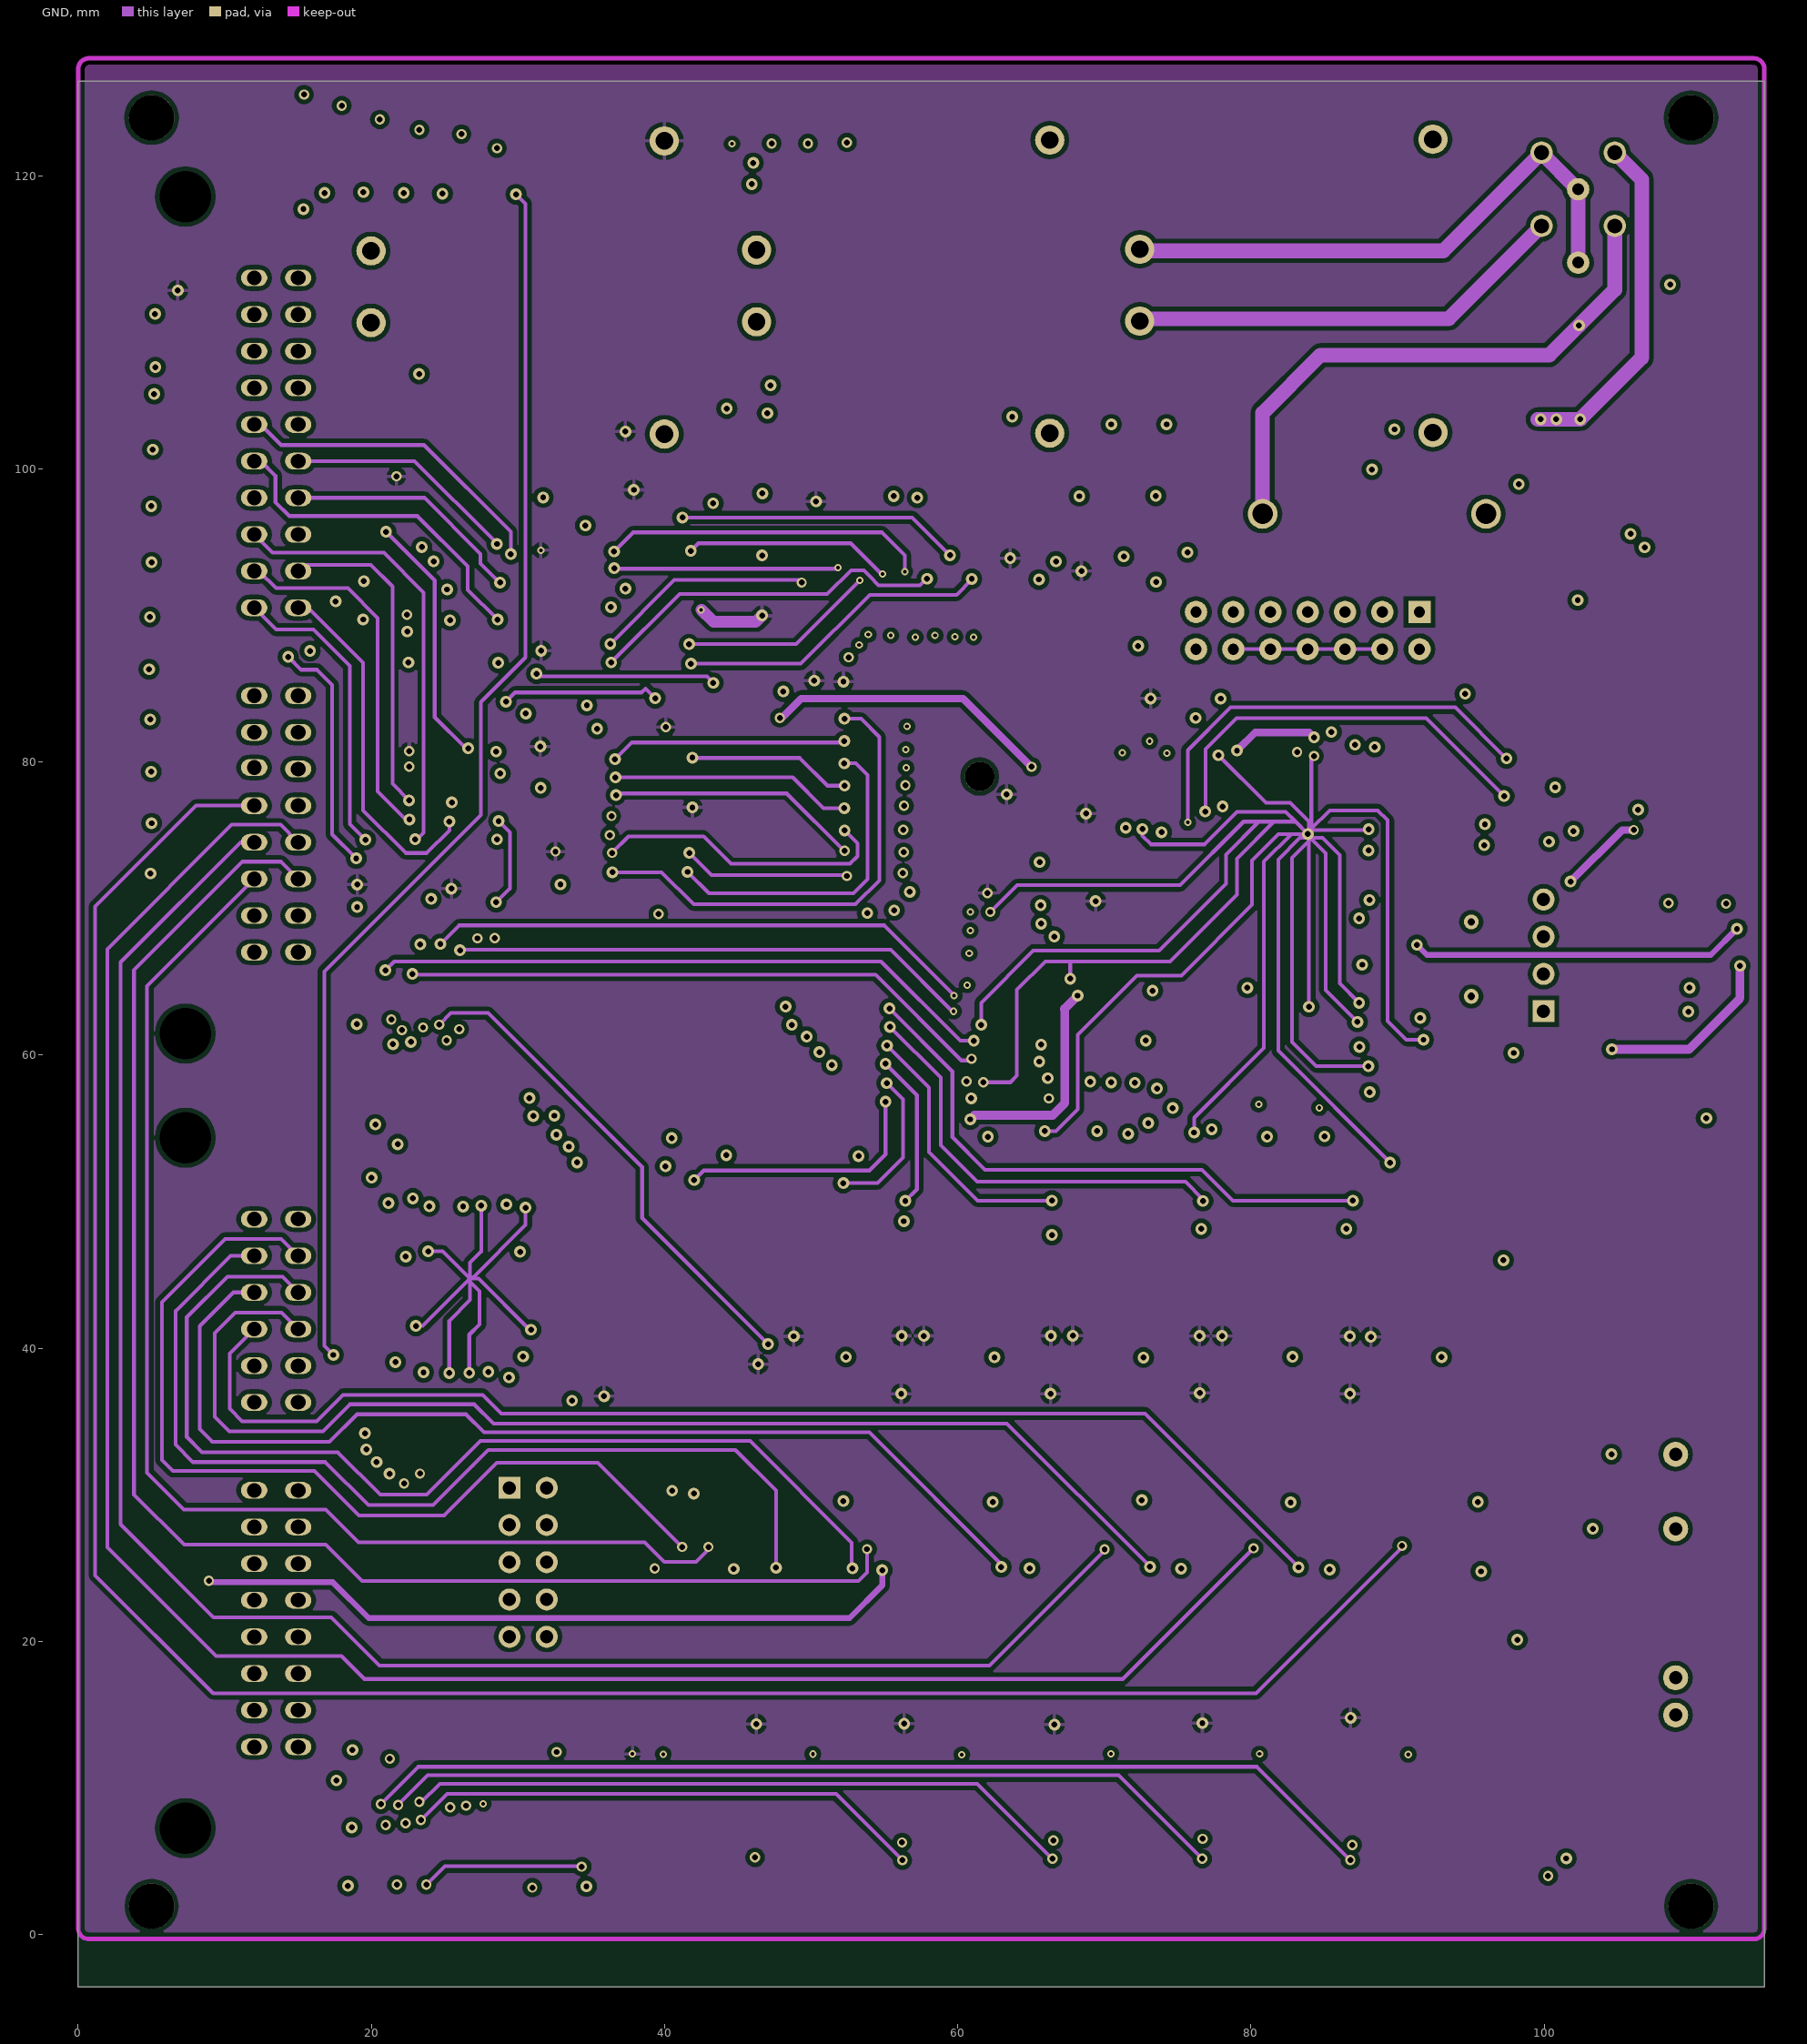
[diagram p0: GND]
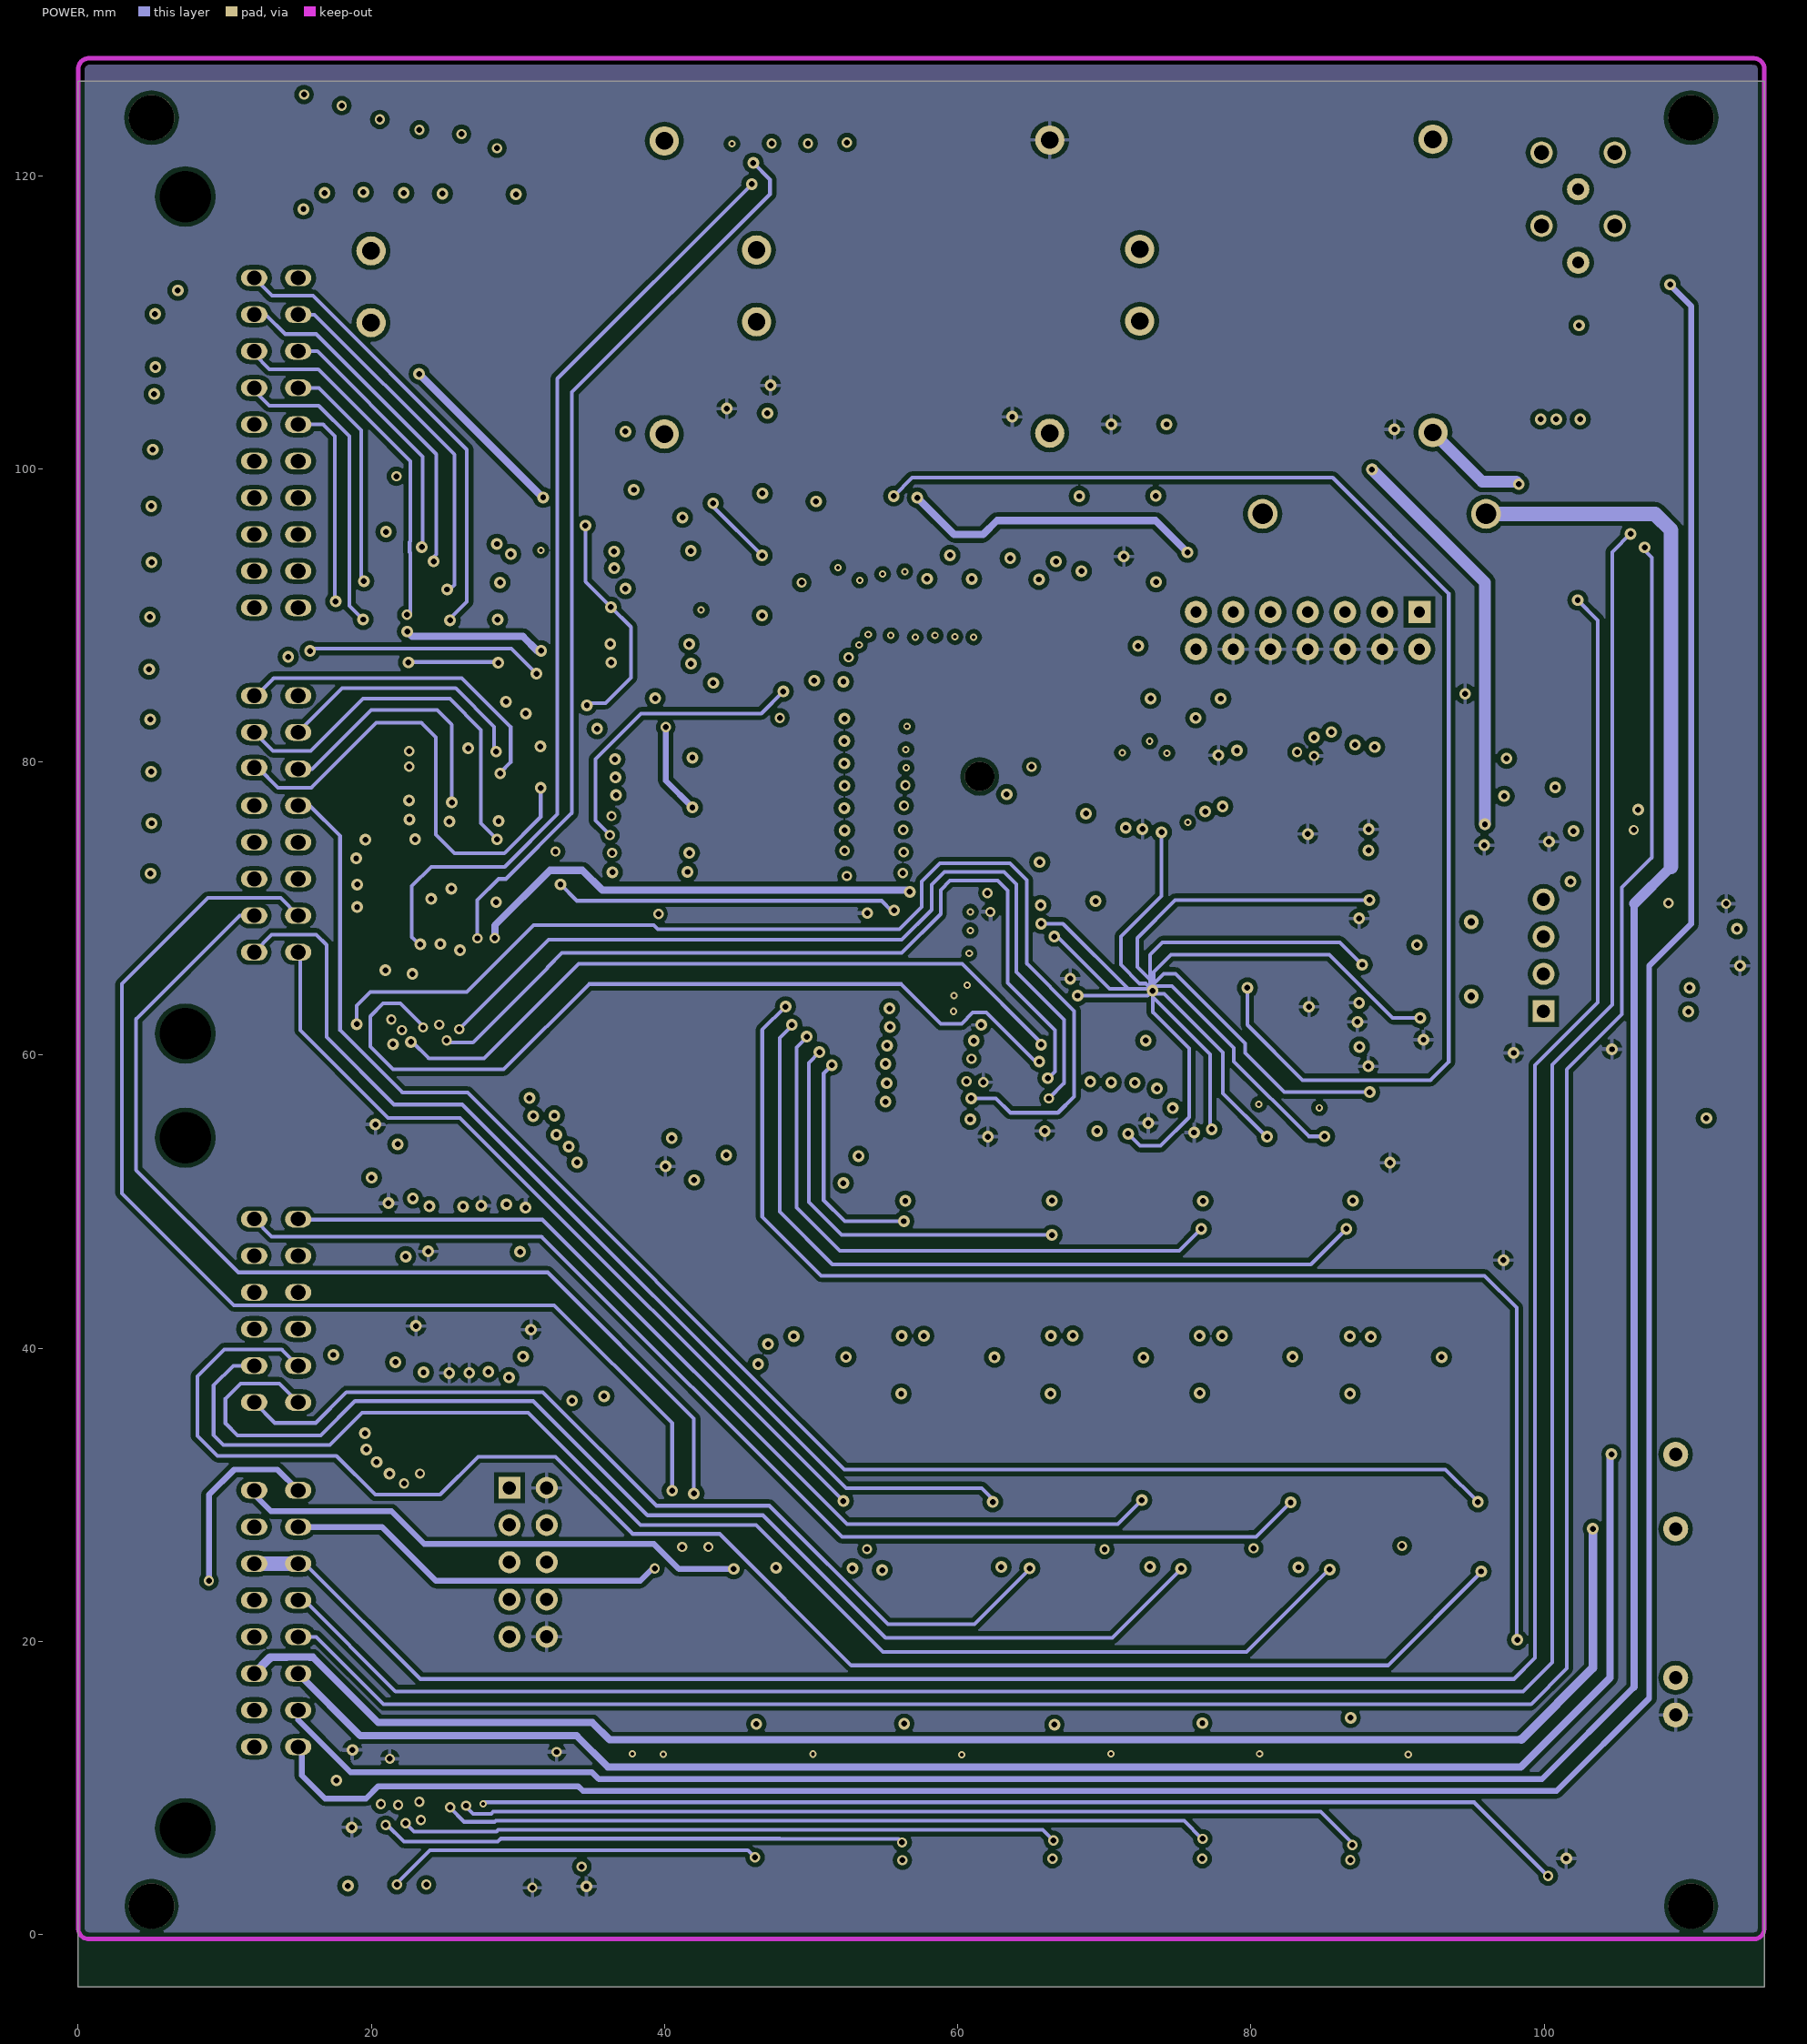
[diagram p1: POWER]
# Altium PCB MISC86180.PCBDOC (part 2 of 9)
## Components (designator, comment, footprint, x,y, rotation, side; value= is the part's Value field where it differs from the comment) (continued)
JC1 "AMP-36P" 36P 15.01,67.022 r180 top locked
JC2 "AMP-28P" 28P 15.01,53.814 r180 top
L1 "Inductor" INDC2012-0805 30.82,71.1 r180 top
L2 "Inductor" CR3225-1210 37.13,65.33 r180 bottom
L3 "Inductor" CR3225-1210 75.71,71.63 r90 top
R1 "Res2" CR1608-0603 56.39,99.27 r180 bottom
R2 "Res2" CR1608-0603 74.39,93.35 r180 bottom
R3 "Res2" CR2012-0805 73.99,67.19 r270 top
R4 "Res2" CR2012-0805 71.17,67.16 r90 top
R5 "Res2" CR1608-0603 92.33,86.05 r180 bottom
R6 "Res2" CR1608-0603 73.122,89.014 r0 bottom
R7 "Res2" CR1608-0603 77.1,84.34 r180 bottom
R8 "Res2" CR1608-0603 84.16,55.53 r180 top
R9 "Res2" CR1608-0603 68.98,60.126 r90 top
R10 "Res2" CR1608-0603 70.504,60.126 r90 top
R11 "Res2" CR1608-0603 72.028,60.126 r90 top
R12 "Res2" CR1608-0603 73.552,60.126 r90 top
R13 "Res2" CR1608-0603 102.04,77.21 r270 top
R14 "Res2" CR1608-0603 103.55,77.21 r90 top
R17 "Res2" CR2012-0805 103.69,99.45 r90 bottom
R18 "Res2" CR2012-0805 103.23,96.48 r180 bottom
R19 "Res2" CR2012-0805 103.134,92.676 r180 bottom
R20 "Res2" CR1608-0603 111.49,86.84 r270 bottom
R21 "Res2" CR1608-0603 110.99,62.02 r90 bottom
R22 "Res2" CR1608-0603 107.92,66 r180 bottom
R23 "Res2" CR1608-0603 111.56,75.08 r90 bottom
R24 "Res2" CR1608-0603 107.87,64.62 r180 bottom
R33 "Res2" CR2012-0805 95.396,49.094 r90 top
R34 "Res2" CR2012-0805 90.316,49.094 r90 top
R35 "Res2" CR2012-0805 84.728,49.094 r90 top
R36 "Res2" CR2012-0805 80.156,49.094 r90 top
R37 "Res2" CR2012-0805 75.076,49.094 r90 top
R38 "Res2" CR2012-0805 69.996,49.094 r90 top
R41 "Res2" CR2012-0805 64.916,49.094 r90 top
R42 "Res2" CR2012-0805 59.836,49.094 r90 top
R43 "Res2" CR2012-0805 54.756,49.094 r90 top
R44 "Res2" CR2012-0805 49.676,49.094 r90 top
R45 "Res2" CR2012-0805 44.596,49.094 r90 top
R46 "Res2" CR2012-0805 39.516,49.094 r90 top
R47 "Res2" CR2012-0805 37.484,49.094 r90 bottom
R48 "Res2" CR2012-0805 42.056,49.094 r90 bottom
R49 "Res2" CR2012-0805 47.644,49.094 r90 bottom
R50 "Res2" CR2012-0805 52.216,49.094 r90 bottom
R51 "Res2" CR2012-0805 57.804,49.094 r90 bottom
R52 "Res2" CR2012-0805 62.376,49.094 r90 bottom
R53 "Res2" CR2012-0805 67.964,49.094 r90 bottom
R54 "Res2" CR2012-0805 72.536,49.094 r90 bottom
R55 "Res2" CR2012-0805 78.124,49.094 r90 bottom
R56 "Res2" CR2012-0805 82.696,49.094 r90 bottom
R57 "Res2" CR2012-0805 88.284,49.094 r90 bottom
R58 "Res2" CR2012-0805 92.856,49.094 r90 bottom
R59 "Res2" CR2012-0805 37.89,3.47 r0 top
R60 "Res2" CR2012-0805 41.8,3.46 r180 top
R61 "Res2" CR2012-0805 47.96,3.52 r0 top
R62 "Res2" CR2012-0805 51.95,3.48 r180 top
R63 "Res2" CR2012-0805 58.42,3.58 r0 top
R64 "Res2" CR2012-0805 62.06,3.53 r180 top
R65 "Res2" CR2012-0805 68.57,3.58 r0 top
R66 "Res2" CR2012-0805 72.27,3.55 r180 top
R67 "Res2" CR2012-0805 78.72,3.57 r0 top
R68 "Res2" CR2012-0805 82.44,3.54 r180 top
R69 "Res2" CR2012-0805 88.93,3.53 r0 top
R70 "Res2" CR2012-0805 92.57,3.52 r180 top
R71 "Res2" CR2012-0805 94.95,3.56 r180 bottom
R72 "Res2" CR2012-0805 91.08,3.49 r0 bottom
R73 "Res2" CR2012-0805 84.85,3.61 r180 bottom
R74 "Res2" CR2012-0805 80.88,3.55 r0 bottom
R75 "Res2" CR2012-0805 74.35,3.57 r180 bottom
R76 "Res2" CR2012-0805 70.7,3.53 r0 bottom
R77 "Res2" CR2012-0805 64.46,3.56 r180 bottom
R78 "Res2" CR2012-0805 60.58,3.54 r0 bottom
R79 "Res2" CR2012-0805 54.03,3.55 r180 bottom
R80 "Res2" CR2012-0805 50.43,3.47 r0 bottom
R81 "Res2" CR2012-0805 43.76,3.51 r180 bottom
R82 "Res2" CR2012-0805 40.23,3.48 r0 bottom
R83 "Res2" CR1608-0603 30.26,33.35 r180 bottom
R84 "Res2" CR1608-0603 26.83,26.77 r270 bottom
R85 "Res2" CR1608-0603 26.83,21.15 r270 bottom
R86 "Res2" CR1608-0603 59.05,65.5 r0 top
R87 "Res2" CR1608-0603 59.05,65.5 r180 bottom
R88 "Res2" CR1608-0603 59.05,67.024 r0 top
R89 "Res2" CR1608-0603 59.05,67.024 r180 bottom
R90 "Res2" CR1608-0603 59.05,68.548 r0 top
R91 "Res2" CR1608-0603 59.05,68.548 r180 bottom
R92 "Res2" CR1608-0603 59.05,70.072 r0 top
R93 "Res2" CR1608-0603 59.05,70.072 r180 bottom
R94 "Res2" CR1608-0603 52.46,120.332 r90 bottom
R95 "Res2" CR1608-0603 49.806,120.302 r90 bottom
R96 "Res2" CR1608-0603 44.628,120.302 r90 bottom
R97 "Res2" CR1608-0603 47.274,120.292 r90 bottom
R98 "Res2" CR1608-0603 15.404,119.704 r90 bottom
R99 "Res2" CR1608-0603 17.99,119.664 r90 bottom
R100 "Res2" CR1608-0603 20.616,119.664 r90 bottom
R101 "Res2" CR1608-0603 23.312,119.664 r90 bottom
R102 "Res2" CR1608-0603 26.168,119.664 r90 bottom
R103 "Res2" CR1608-0603 28.574,119.674 r90 bottom
R104 "Res2" CR2012-0805 105.37,17.51 r180 bottom
R105 "Res2" CR1608-0603 30.66,73.43 r180 top
R106 "Res2" CR2012-0805 3.05,114.03 r180 bottom
R107 "Res2" CR2012-0805 7.66,110.54 r180 bottom
R108 "Res2" CR2012-0805 3.079,110.528 r180 bottom
R109 "Res2" CR2012-0805 7.539,106.828 r180 bottom
R110 "Res2" CR2012-0805 3.12,106.95 r180 bottom
R111 "Res2" CR2012-0805 7.54,103.29 r180 bottom
R112 "Res2" CR2012-0805 3.12,103.27 r180 bottom
R113 "Res2" CR2012-0805 7.44,99.3 r180 bottom
R114 "Res2" CR2012-0805 3,99.44 r180 bottom
R115 "Res2" CR2012-0805 7.4,95.52 r180 bottom
R116 "Res2" CR2012-0805 2.96,95.52 r180 bottom
R117 "Res2" CR2012-0805 7.33,91.94 r180 bottom
R118 "Res2" CR2012-0805 2.87,91.94 r180 bottom
R119 "Res2" CR2012-0805 7.32,88.1 r180 bottom
R120 "Res2" CR2012-0805 2.89,88.19 r180 bottom
R121 "Res2" CR2012-0805 7.32,84.51 r180 bottom
R122 "Res2" CR2012-0805 2.91,84.51 r180 bottom
R123 "Res2" CR2012-0805 7.24,81.14 r180 bottom
R124 "Res2" CR2012-0805 2.94,81.12 r180 bottom
R125 "Res2" CR2012-0805 7.28,77.59 r180 bottom
R126 "Res2" CR2012-0805 2.92,77.6 r180 bottom
R127 "Res2" CR2012-0805 7.289,74.128 r180 bottom
R128 "Res2" CR2012-0805 2.96,74.18 r180 bottom
R129 "Res2" CR2012-0805 7.28,70.66 r180 bottom
R130 "Res2" CR2012-0805 2.944,70.636 r180 bottom
R131 "Res2" CR2012-0805 46.668,83.942 r90 top
R132 "Res2" CR2012-0805 46.668,88.006 r90 top
R133 "Res2" CR2012-0805 46.668,96.134 r270 top
R134 "Res2" CR2012-0805 46.668,92.07 r270 top
R136 "Res2" CR2012-0805 32.602,96.144 r0 top
R137 "Res2" CR1608-0603 50.302,94.954 r270 top
R138 "Res2" CR1608-0603 50.302,90.382 r90 top
R139 "Res2" CR1608-0603 51.826,94.954 r270 top
R140 "Res2" CR1608-0603 51.826,90.382 r90 top
R141 "Res2" CR1608-0603 53.35,94.954 r270 top
R142 "Res2" CR1608-0603 53.35,90.382 r90 top
R143 "Res2" CR1608-0603 54.874,94.954 r270 top
R144 "Res2" CR1608-0603 54.874,90.382 r90 top
R145 "Res2" CR1608-0603 56.398,94.954 r270 top
R146 "Res2" CR1608-0603 56.398,90.382 r90 top
R147 "Res2" CR1608-0603 57.922,94.954 r270 top
R148 "Res2" CR1608-0603 57.922,90.382 r90 top
R149 "Res2" CR1608-0603 59.446,94.954 r270 top
R150 "Res2" CR1608-0603 59.446,90.382 r90 top
R151 "Res2" CR1608-0603 60.97,94.954 r270 top
R152 "Res2" CR1608-0603 60.97,90.382 r90 top
R153 "Res2" CR1608-0603 50.018,82.97 r0 top
R154 "Res2" CR1608-0603 54.59,82.97 r180 top
R155 "Res2" CR1608-0603 50.018,81.446 r0 top
R156 "Res2" CR1608-0603 54.59,81.446 r180 top
R157 "Res2" CR1608-0603 50.018,79.922 r0 top
R158 "Res2" CR1608-0603 54.59,79.922 r180 top
R159 "Res2" CR1608-0603 50.018,78.398 r0 top
R160 "Res2" CR1608-0603 54.59,78.398 r180 top
R161 "Res2" CR1608-0603 50.018,76.874 r0 top
R162 "Res2" CR1608-0603 54.59,76.874 r180 top
R163 "Res2" CR1608-0603 50.018,75.35 r0 top
R164 "Res2" CR1608-0603 54.59,75.35 r180 top
R165 "Res2" CR1608-0603 50.018,73.826 r0 top
R166 "Res2" CR1608-0603 54.59,73.826 r180 top
R167 "Res2" CR1608-0603 50.018,72.302 r0 top
R168 "Res2" CR1608-0603 54.59,72.302 r180 top
R170 "Res2" CR2012-0805 34.574,68.01 r0 top
R171 "Res2" CR2012-0805 38.638,68.01 r0 top
R172 "Res2" CR2012-0805 38.638,68.01 r180 bottom
R173 "Res2" CR2012-0805 34.62,68.07 r180 bottom
R180 "Res2" CR2012-0805 67.52,88.02 r0 bottom
R181 "Res2" CR1608-0603 74.53,82.32 r90 top
S1 "AQW214" AQW214 96.92,44.522 r270 top
S2 "AQW214" AQW214 86.76,44.522 r270 top
S3 "AQW214" AQW214 76.6,44.522 r270 top
S4 "AQW214" AQW214 66.44,44.522 r270 top
S5 "AQW214" AQW214 56.28,44.522 r270 top
S6 "AQW214" AQW214 46.12,44.522 r270 top
S7 "AQW214" AQW214 35.96,44.522 r270 bottom
S8 "AQW214" AQW214 46.12,44.522 r270 bottom
S9 "AQW214" AQW214 56.28,44.522 r270 bottom
S10 "AQW214" AQW214 66.44,44.522 r270 bottom
S11 "AQW214" AQW214 76.6,44.522 r270 bottom
S12 "AQW214" AQW214 86.76,44.522 r270 bottom
S13 "AQW214" AQW214 36,7.154 r90 top
S14 "AQW214" AQW214 46.16,7.154 r90 top
S15 "AQW214" AQW214 56.32,7.154 r90 top
S16 "AQW214" AQW214 66.48,7.154 r90 top
S17 "AQW214" AQW214 76.64,7.154 r90 top
S18 "AQW214" AQW214 86.8,7.154 r90 top
S19 "AQW214" AQW214 96.96,7.154 r90 bottom
S20 "AQW214" AQW214 86.8,7.154 r90 bottom
S21 "AQW214" AQW214 76.64,7.154 r90 bottom
S22 "AQW214" AQW214 66.48,7.154 r90 bottom
S23 "AQW214" AQW214 56.32,7.154 r90 bottom
S24 "AQW214" AQW214 46.16,7.154 r90 bottom
SW1 "SW-PB" SW_RESET 72.574,98.916 r0 top
TVS1 "1.5KE30A" SB560 96.03,96.91 r180 top
U1 "1205" DCDC_5W 4.99,125.8 r0 top
U2 "1205" DCDC_5W 31.28,125.86 r0 top
U3 "1205" DCDC_5W 57.414,125.91 r0 top locked
U4 "TPS75733" 75733 64.514,116.158 r180 bottom
U5 "TPS76801Q" D008 79.04,64.3 r90 top
U6 "TPS75733" 75733 38.314,116.148 r180 bottom
U7 "TPS75733" 75733 90.434,116.258 r180 bottom
U8 "TPS3823-33" DBV005 74.606,96.376 r90 bottom
U9 "TMS320F283XXPGF_23" QFP176NEW 63.9,55.046 r90 bottom locked
U10 "SN74CBTD3384DBLE" DBQ024 96.53,79.26 r90 top
U11 "ZJYS-81R5-2PL" ZJYS 112.278,93.176 r90 bottom
U13 "SN65HVD251" D008 107.86,85.05 r180 bottom
U15 "HCPL063" SO-G8 107.608,58.312 r180 bottom
U16 "HCPL063" SO-G8 108.07,71.19 r180 bottom
U19 "EPM240T100C5N" TQFP100 26.816,44.014 r90 top locked
U20 "SN74CBTD3384DBLE" DBQ024 23.686,61.458 r180 bottom
U21 "SN74LVC4245PW" WSO24 48.792,61.314 r270 bottom
U22 "SN74LVC4245PW" WSO24 48.792,61.314 r90 top
U23 "SN74LVC4245PW" WSO24 25.71,9.88 r0 top
U24 "SN74LVC4245PW" WSO24 25.704,9.892 r180 bottom locked
U25 "MAX4619" SO16 20.998,94.802 r0 top
U26 "MAX4619" SO16 26.934,79.792 r180 bottom
U27 "MAX4619" SO16 20.941,79.79 r0 top
U28 "MAX4619" SO16 26.991,94.8 r180 bottom
U29 "OPA4350" 751A-02 37.174,90.556 r270 top
U30 "OPA4350" 751A-02 37.174,90.556 r90 bottom
U31 "OPA4350" 751A-02 37.134,76.37 r270 top
U32 "OPA4350" 751A-02 37.134,76.37 r90 bottom
U34 "ADR420" SO-G8 66.17,92.908 r180 top
U35 "AQZ102" AQZ102 107.93,13.71 r90 top
Y1 "30M" Oscillator 95.02,64.005 r270 top

## Footprints (in the part's own frame and the unit in brackets; to place one, negate y for a bottom-side part, rotate by r counter-clockwise, add the part's x,y. Pads: shape width x height; smd on the part's side, far side on the other; paste and mask are expansions set on the pad)
28P [mm]
  round 1.8 hole 3.5: 0(7.7,46.55) 0(7.7,-0.55)
  oval 1.8x1.143 hole 1: 3(0,5) 4(0,7.5) 5(0,10) 6(0,12.5) 7(0,15) 8(0,17.5) 9(0,23.5) 10(0,26) 13(3,5) 14(3,7.5) 15(3,10) 16(3,12.5) 17(3,15) 18(3,17.5) 19(3,23.5) 20(3,26) 21(0,28.5) 22(0,31) 23(0,33.5) 24(0,36) 25(0,38.5) 26(0,41) 29(3,28.5) 30(3,31) 31(3,33.5) 32(3,36) 33(3,38.5) 34(3,41)
  silkscreen extent 4.4,-3.8 11.68,49.8
36P [mm]
  round 1.8 hole 3.5: 0(7.7,5.55) 0(7.7,-51.55)
  oval 1.8x1.143 hole 1: 1(0,-46) 2(0,-43.5) 3(0,-41) 4(0,-38.5) 5(0,-36) 6(0,-33.5) 7(0,-31) 8(0,-28.5) 9(0,-26) 10(0,-23.5) 11(3,-46) 12(3,-43.5) 13(3,-41) 14(3,-38.5) 15(3,-36) 16(3,-33.5) 17(3,-31) 18(3,-28.5) 19(3,-26) 20(3,-23.5) 21(0,-17.5) 22(0,-15) 23(0,-12.5) 24(0,-10) 25(0,-7.5) 26(0,-5) 27(0,-2.5) 28(0,0) 29(3,-17.5) 30(3,-15) 31(3,-12.6) 32(3,-10) 33(3,-7.5) 34(3,-5) 35(3,-2.5) 36(3,0)
  silkscreen extent 4.4,-54.8 11.68,8.8
751A-02 [mm]
  rect 0.6x2.2 smd: 1(-3.805,-2.62) 2(-2.535,-2.62) 3(-1.265,-2.62) 4(0.005,-2.62) 5(1.275,-2.62) 6(2.545,-2.62) 7(3.815,-2.62) 8(3.815,2.63) 9(2.545,2.63) 10(1.275,2.63) 11(0.005,2.63) 12(-1.265,2.63) 13(-2.535,2.63) 14(-3.805,2.63)
  silkscreen extent -4.78,-2.74 4.38,1.13
1206 [mil]
  rect 60x60 smd: 1(0.28,-0.39) 2(135.28,-0.39)
  silkscreen extent -50,-50 185,50
75733 [mm]
  rect 1.05x2.1 smd: 1(2.167,-13.593) 2(3.867,-13.593) 3(5.567,-13.593) 4(7.267,-13.593) 5(8.967,-13.593)
  rect 11.176x11 smd: 6(5.605,-4.045)
  silkscreen extent 0,-14.54 11.13,1.43
AK_1B [mil]
  rect 100x60 smd: 1(0,-170) 2(0,0)
  silkscreen extent -82,-134 72,-36
AQW214 [mil]
  rect 100x45 smd: 1(-50,-60) 2(-50,-155) 3(-50,-250) 4(-50,-345) 5(300,-345) 6(300,-250) 7(300,-155) 8(300,-60)
  silkscreen extent 0,-400 250,0